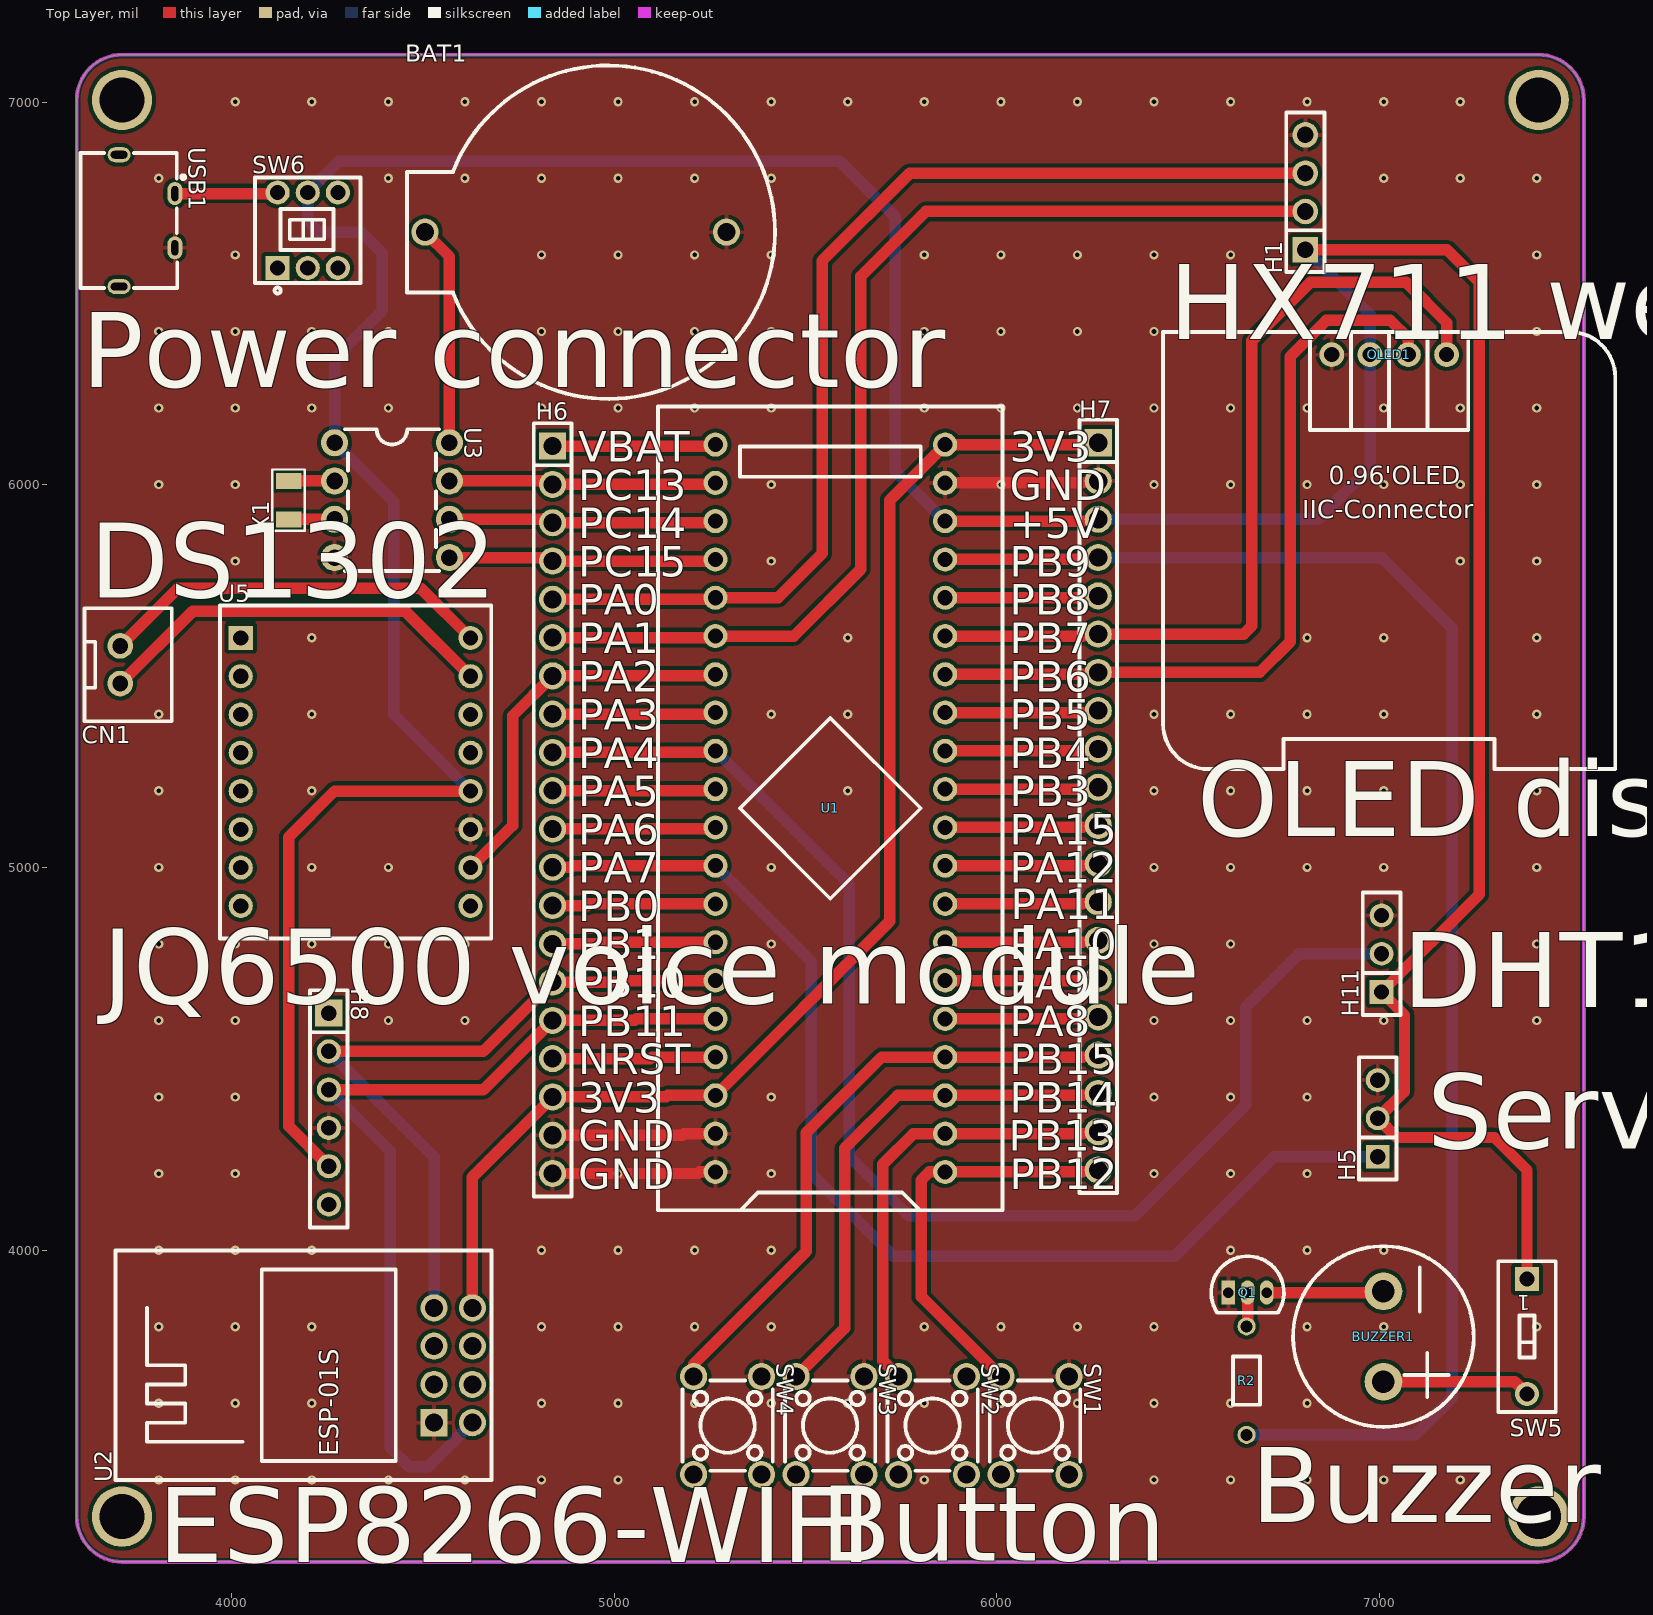
[diagram p0: Top Layer view]
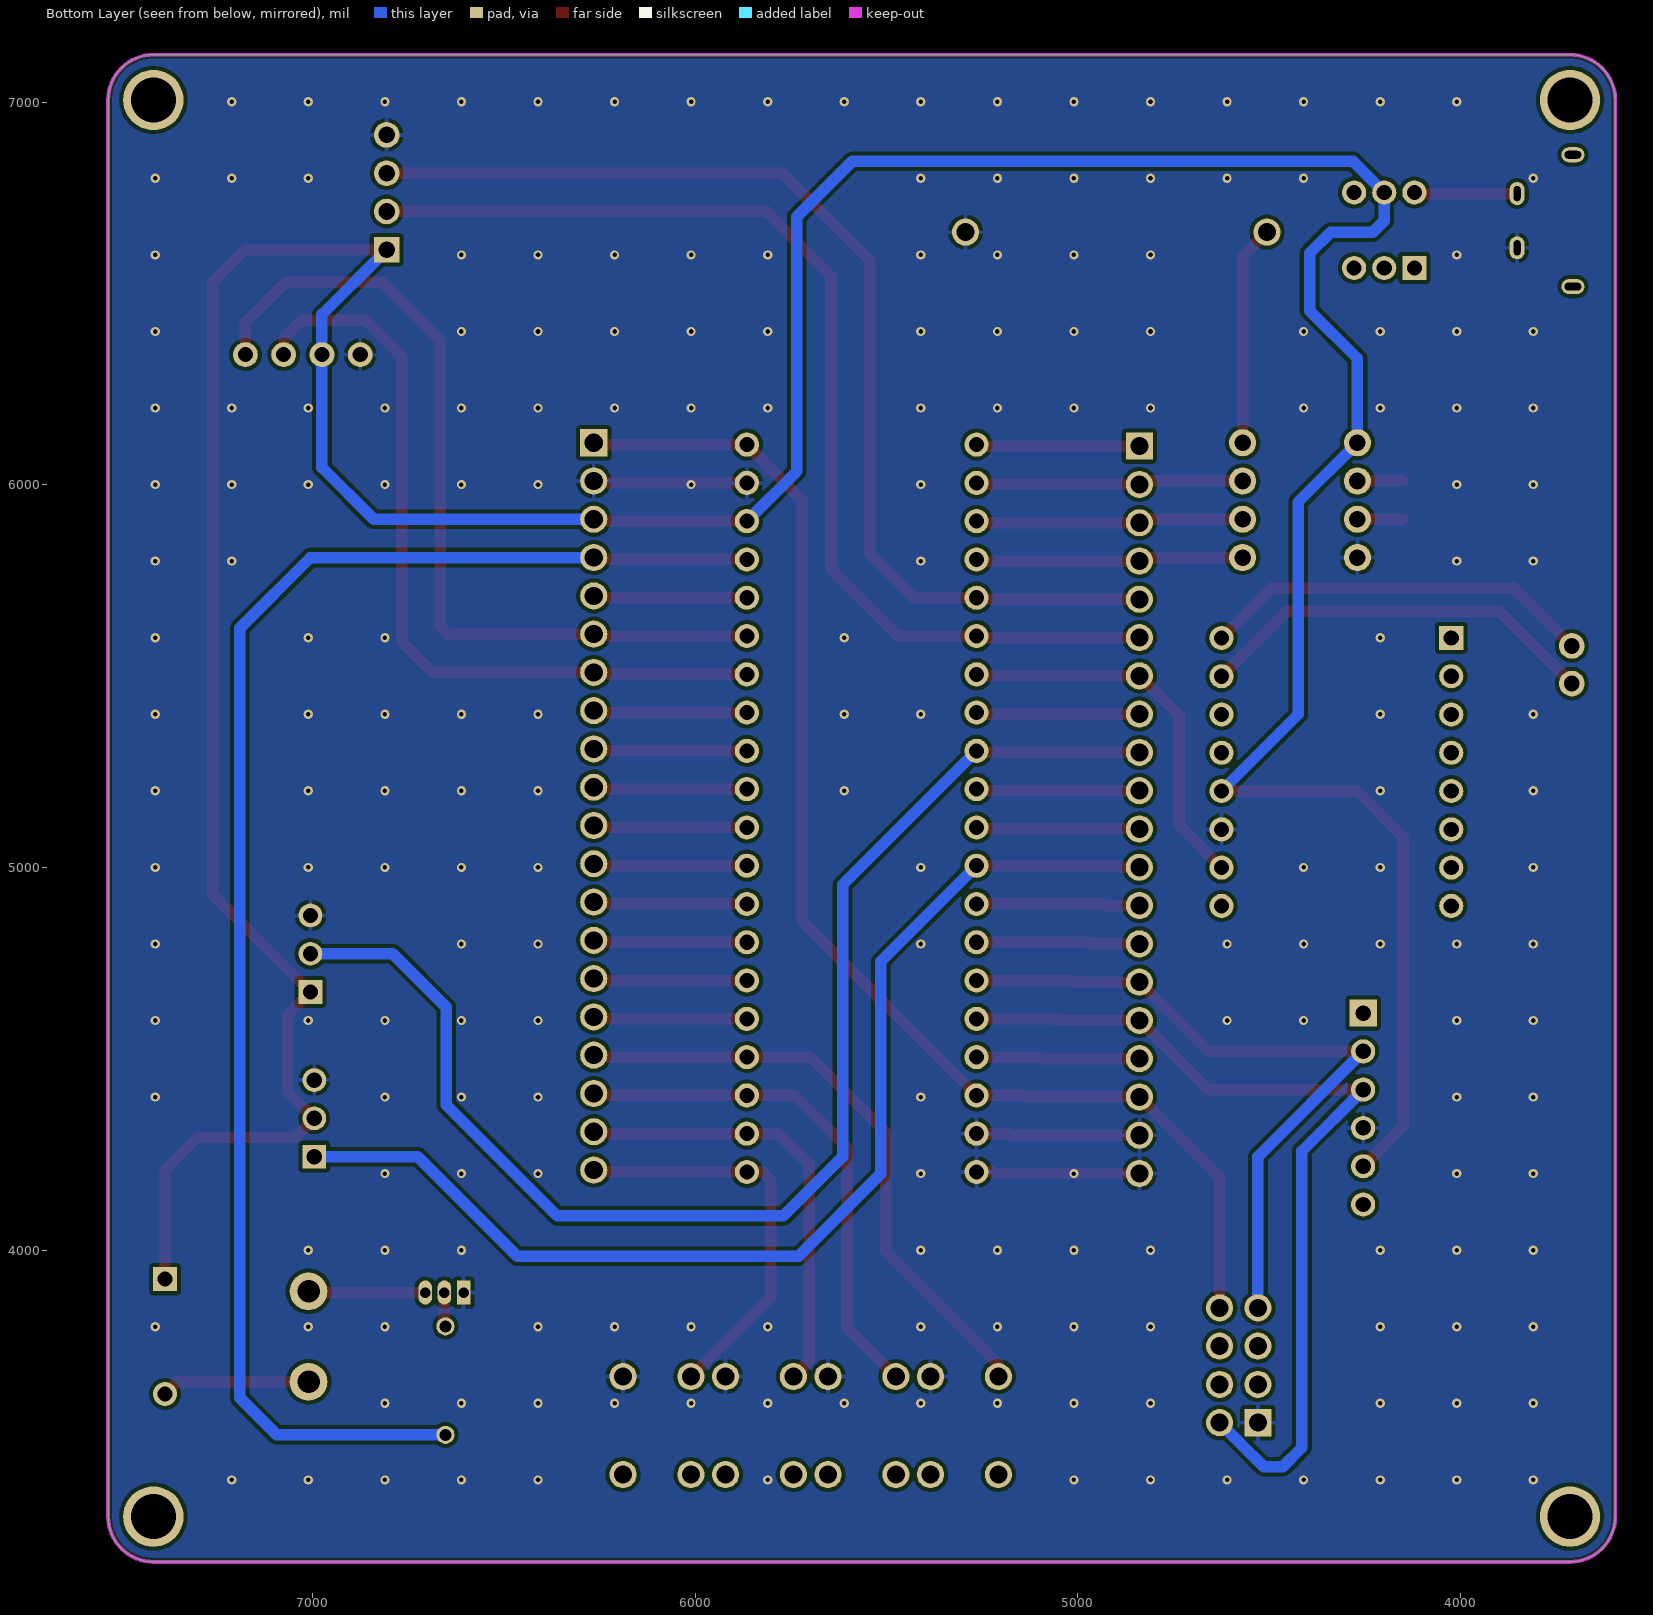
[diagram p1: Bottom Layer view, seen from below]
# Altium PCB MISC51988.pcbdoc
Units mil, origin at the board's own origin, x right, y up, seen from the top; angles counter-clockwise.
Board outline 3937.01 x 3937.01 mil, 2 copper layers (Top Layer, Bottom Layer), stack 62.206 mil thick; 24 components, 46 nets, 177 pads, 198 vias.

## Layer stack, top to bottom
Top Solder Mask Layer: solder mask 0.394, Dk 3.3
Top Layer: signal copper 1.379
Dielectric1: surface 59.449, FR4, Dk 4.5
Bottom Layer: signal copper 1.378
Bottom Solder Mask Layer: solder mask 0.394, Dk 3.3

## Board outline
3714.61,7123.5 ccw(c3714.61,7005.39) 3596.5,7005.39 3596.5,3304.61 ccw(c3714.61,3304.61) 3714.61,3186.5 7415.39,3186.5 ccw(c7415.39,3304.61) 7533.5,3304.61 7533.5,7005.39 ccw(c7415.39,7005.39) 7415.39,7123.5 3714.61,7123.5

## Design rules (kind name [scope] priority, off if disabled: settings)
BoardOutlineClearance copperThickness2oz_1 [All] p2 off: genericclearance=7.99 ignorepadtopadclearanceinfootprint=FALSE except(0: Arc-SplitContinuation Track-SplitContinuation SMDPad-SplitContinuation THPad-SplitContinuation Via-SplitContinuation Fill-SplitContinuation Region-SplitContinuation Poly-SplitContinuation Text-SplitContinuation Hole-SplitContinuation; 5.98: Arc-CutoutEdge Track-CutoutEdge SMDPad-CutoutEdge THPad-CutoutEdge Via-CutoutEdge Text-CutoutEdge; 6.9: Hole-OutlineEdge Hole-CutoutEdge; 10: Poly-OutlineEdge Poly-CutoutEdge; 11.81: Arc-OutlineEdge Track-OutlineEdge SMDPad-OutlineEdge THPad-OutlineEdge Via-OutlineEdge Fill-OutlineEdge Region-OutlineEdge Text-OutlineEdge Fill-CutoutEdge Region-CutoutEdge)
BoardOutlineClearance Plane_innerPlane_1 [All] p4 off: genericclearance=4.02 ignorepadtopadclearanceinfootprint=FALSE except(0: Arc-SplitContinuation Track-SplitContinuation SMDPad-SplitContinuation THPad-SplitContinuation Via-SplitContinuation Fill-SplitContinuation Region-SplitContinuation Poly-SplitContinuation Text-SplitContinuation Hole-SplitContinuation; 5.98: Arc-CutoutEdge Track-CutoutEdge SMDPad-CutoutEdge THPad-CutoutEdge Via-CutoutEdge Text-CutoutEdge; 6.9: Hole-OutlineEdge Hole-CutoutEdge; 10: Poly-OutlineEdge Poly-CutoutEdge; 11.81: Arc-OutlineEdge Track-OutlineEdge SMDPad-OutlineEdge THPad-OutlineEdge Via-OutlineEdge Fill-OutlineEdge Region-OutlineEdge Text-OutlineEdge Fill-CutoutEdge Region-CutoutEdge)
BoardOutlineClearance Copper_copperRegion_1 [All] p6 off: genericclearance=4.02 ignorepadtopadclearanceinfootprint=FALSE except(0: Arc-SplitContinuation Track-SplitContinuation SMDPad-SplitContinuation THPad-SplitContinuation Via-SplitContinuation Fill-SplitContinuation Region-SplitContinuation Poly-SplitContinuation Text-SplitContinuation Hole-SplitContinuation; 5.98: Arc-CutoutEdge Track-CutoutEdge SMDPad-CutoutEdge THPad-CutoutEdge Via-CutoutEdge Text-CutoutEdge; 6.9: Hole-OutlineEdge Hole-CutoutEdge; 10: Poly-OutlineEdge Poly-CutoutEdge; 11.81: Arc-OutlineEdge Track-OutlineEdge SMDPad-OutlineEdge THPad-OutlineEdge Via-OutlineEdge Fill-OutlineEdge Region-OutlineEdge Text-OutlineEdge Fill-CutoutEdge Region-CutoutEdge)
BoardOutlineClearance Copper_copperRegion_copperThickness1oz_1 [All] p8 off: genericclearance=4.02 ignorepadtopadclearanceinfootprint=FALSE except(0: Arc-SplitContinuation Track-SplitContinuation SMDPad-SplitContinuation THPad-SplitContinuation Via-SplitContinuation Fill-SplitContinuation Region-SplitContinuation Poly-SplitContinuation Text-SplitContinuation Hole-SplitContinuation; 5.98: Arc-CutoutEdge Track-CutoutEdge SMDPad-CutoutEdge THPad-CutoutEdge Via-CutoutEdge Text-CutoutEdge; 6.9: Hole-OutlineEdge Hole-CutoutEdge; 10: Poly-OutlineEdge Poly-CutoutEdge; 11.81: Arc-OutlineEdge Track-OutlineEdge SMDPad-OutlineEdge THPad-OutlineEdge Via-OutlineEdge Fill-OutlineEdge Region-OutlineEdge Text-OutlineEdge Fill-CutoutEdge Region-CutoutEdge)
BoardOutlineClearance Copper_copperRegion_Copper_copperRegion_1 [All] p10 off: genericclearance=4.02 ignorepadtopadclearanceinfootprint=FALSE except(0: Arc-SplitContinuation Track-SplitContinuation SMDPad-SplitContinuation THPad-SplitContinuation Via-SplitContinuation Fill-SplitContinuation Region-SplitContinuation Poly-SplitContinuation Text-SplitContinuation Hole-SplitContinuation; 5.98: Arc-CutoutEdge Track-CutoutEdge SMDPad-CutoutEdge THPad-CutoutEdge Via-CutoutEdge Text-CutoutEdge; 6.9: Hole-OutlineEdge Hole-CutoutEdge; 10: Poly-OutlineEdge Poly-CutoutEdge; 11.81: Arc-OutlineEdge Track-OutlineEdge SMDPad-OutlineEdge THPad-OutlineEdge Via-OutlineEdge Fill-OutlineEdge Region-OutlineEdge Text-OutlineEdge Fill-CutoutEdge Region-CutoutEdge)
BoardOutlineClearance copperThickness1oz_1 [All] p12: genericclearance=4.02 ignorepadtopadclearanceinfootprint=FALSE except(0: Arc-SplitContinuation Track-SplitContinuation SMDPad-SplitContinuation THPad-SplitContinuation Via-SplitContinuation Fill-SplitContinuation Region-SplitContinuation Poly-SplitContinuation Text-SplitContinuation Hole-SplitContinuation; 5.98: Arc-CutoutEdge Track-CutoutEdge SMDPad-CutoutEdge THPad-CutoutEdge Via-CutoutEdge Text-CutoutEdge; 6.9: Hole-OutlineEdge Hole-CutoutEdge; 10: Poly-OutlineEdge Poly-CutoutEdge; 11.81: Arc-OutlineEdge Track-OutlineEdge SMDPad-OutlineEdge THPad-OutlineEdge Via-OutlineEdge Fill-OutlineEdge Region-OutlineEdge Text-OutlineEdge Fill-CutoutEdge Region-CutoutEdge)
Clearance copperThickness2oz [All] p1 off: gap=7.99 ignorepadtopadclearanceinfootprint=FALSE except(5.98: SMDPad-Track SMDPad-SMDPad THPad-Track SMDPad-THPad THPad-THPad Track-Via SMDPad-Via THPad-Via Via-Via Fill-SMDPad Region-SMDPad Fill-THPad Region-THPad Fill-Via Region-Via Fill-Fill Fill-Region Region-Region Arc-Track Arc-SMDPad Arc-THPad Arc-Via Fill-Arc Region-Arc Arc-Arc Text-Track SMDPad-Text Text-THPad Text-Via Fill-Text Region-Text Arc-Text Text-Text; 6.9: Hole-Track Hole-SMDPad Hole-THPad Hole-Via Fill-Hole Region-Hole Hole-Arc Hole-Text; 10: Poly-Track Poly-SMDPad Poly-THPad Poly-Via Poly-Fill Poly-Region Poly-Poly Poly-Arc Poly-Text Poly-Hole; 11.81: Fill-Track Region-Track)
Clearance Plane_innerPlane [All] p3 off: gap=4.02 ignorepadtopadclearanceinfootprint=FALSE except(5.98: SMDPad-Track SMDPad-SMDPad THPad-Track SMDPad-THPad THPad-THPad Track-Via SMDPad-Via THPad-Via Via-Via Fill-SMDPad Region-SMDPad Fill-THPad Region-THPad Fill-Via Region-Via Fill-Fill Fill-Region Region-Region Arc-Track Arc-SMDPad Arc-THPad Arc-Via Fill-Arc Region-Arc Arc-Arc Text-Track SMDPad-Text Text-THPad Text-Via Fill-Text Region-Text Arc-Text Text-Text; 6.9: Hole-Track Hole-SMDPad Hole-THPad Hole-Via Fill-Hole Region-Hole Hole-Arc Hole-Text; 10: Poly-Track Poly-SMDPad Poly-THPad Poly-Via Poly-Fill Poly-Region Poly-Poly Poly-Arc Poly-Text Poly-Hole; 11.81: Fill-Track Region-Track)
Clearance Copper_copperRegion [All] p5 off: gap=4.02 ignorepadtopadclearanceinfootprint=FALSE except(5.98: SMDPad-Track SMDPad-SMDPad THPad-Track SMDPad-THPad THPad-THPad Track-Via SMDPad-Via THPad-Via Via-Via Fill-SMDPad Region-SMDPad Fill-THPad Region-THPad Fill-Via Region-Via Fill-Fill Fill-Region Region-Region Arc-Track Arc-SMDPad Arc-THPad Arc-Via Fill-Arc Region-Arc Arc-Arc Text-Track SMDPad-Text Text-THPad Text-Via Fill-Text Region-Text Arc-Text Text-Text; 6.9: Hole-Track Hole-SMDPad Hole-THPad Hole-Via Fill-Hole Region-Hole Hole-Arc Hole-Text; 10: Poly-Track Poly-SMDPad Poly-THPad Poly-Via Poly-Fill Poly-Region Poly-Poly Poly-Arc Poly-Text Poly-Hole; 11.81: Fill-Track Region-Track)
Clearance Copper_copperRegion_copperThickness1oz [All] p7 off: gap=4.02 ignorepadtopadclearanceinfootprint=FALSE except(5.98: SMDPad-Track SMDPad-SMDPad THPad-Track SMDPad-THPad THPad-THPad Track-Via SMDPad-Via THPad-Via Via-Via Fill-SMDPad Region-SMDPad Fill-THPad Region-THPad Fill-Via Region-Via Fill-Fill Fill-Region Region-Region Arc-Track Arc-SMDPad Arc-THPad Arc-Via Fill-Arc Region-Arc Arc-Arc Text-Track SMDPad-Text Text-THPad Text-Via Fill-Text Region-Text Arc-Text Text-Text; 6.9: Hole-Track Hole-SMDPad Hole-THPad Hole-Via Fill-Hole Region-Hole Hole-Arc Hole-Text; 10: Poly-Track Poly-SMDPad Poly-THPad Poly-Via Poly-Fill Poly-Region Poly-Poly Poly-Arc Poly-Text Poly-Hole; 11.81: Fill-Track Region-Track)
Clearance Copper_copperRegion_Copper_copperRegion [All] p9 off: gap=4.02 ignorepadtopadclearanceinfootprint=FALSE except(5.98: SMDPad-Track SMDPad-SMDPad THPad-Track SMDPad-THPad THPad-THPad Track-Via SMDPad-Via THPad-Via Via-Via Fill-SMDPad Region-SMDPad Fill-THPad Region-THPad Fill-Via Region-Via Fill-Fill Fill-Region Region-Region Arc-Track Arc-SMDPad Arc-THPad Arc-Via Fill-Arc Region-Arc Arc-Arc Text-Track SMDPad-Text Text-THPad Text-Via Fill-Text Region-Text Arc-Text Text-Text; 6.9: Hole-Track Hole-SMDPad Hole-THPad Hole-Via Fill-Hole Region-Hole Hole-Arc Hole-Text; 10: Poly-Track Poly-SMDPad Poly-THPad Poly-Via Poly-Fill Poly-Region Poly-Poly Poly-Arc Poly-Text Poly-Hole; 11.81: Fill-Track Region-Track)
Clearance copperThickness1oz [All] p11: gap=4.02 ignorepadtopadclearanceinfootprint=FALSE except(5.98: SMDPad-Track SMDPad-SMDPad THPad-Track SMDPad-THPad THPad-THPad Track-Via SMDPad-Via THPad-Via Via-Via Fill-SMDPad Region-SMDPad Fill-THPad Region-THPad Fill-Via Region-Via Fill-Fill Fill-Region Region-Region Arc-Track Arc-SMDPad Arc-THPad Arc-Via Fill-Arc Region-Arc Arc-Arc Text-Track SMDPad-Text Text-THPad Text-Via Fill-Text Region-Text Arc-Text Text-Text; 6.9: Hole-Track Hole-SMDPad Hole-THPad Hole-Via Fill-Hole Region-Hole Hole-Arc Hole-Text; 10: Poly-Track Poly-SMDPad Poly-THPad Poly-Via Poly-Fill Poly-Region Poly-Poly Poly-Arc Poly-Text Poly-Hole; 11.81: Fill-Track Region-Track)
DiffPairsRouting differentialPair [All] p1: maxlimit=6 minlimit=6 mostfreqgap=6 toplayer_minwidth=5 toplayer_prefwidth=10 toplayer_maxwidth=100 toplayer_mingap=6 toplayer_prefgap=6 toplayer_maxgap=6 bottomlayer_minwidth=5 bottomlayer_prefwidth=10 bottomlayer_maxwidth=100 bottomlayer_mingap=6 bottomlayer_prefgap=6 bottomlayer_maxgap=6 maxuncoupledlength=10
HoleToHoleClearance otherClearance [All] p1: gap=11.81 allowstackedmicrovias=TRUE
Length netLength [All] p1: minlimit=0 maxlimit=0
PasteMaskExpansion pasteMaskExpansion [All] p1: expansion=0
PlaneConnect innerPlane [All] p1: planeconnectstyle=Relief reliefexpansion=20 reliefentries=4 reliefconductorwidth=10 reliefairgap=10
PolygonConnect copperRegion_copperThickness1oz [All] p1 off: connectstyle=Relief reliefconductorwidth=10 reliefentries=4 polygonreliefangle="90 Angle" airgapwidth=10 via.connectstyle=Relief via.reliefconductorwidth=10 via.reliefentries=4 via.polygonreliefangle="90 Angle" via.airgapwidth=10
PolygonConnect copperRegion_Copper_copperRegion [All] p2 off: connectstyle=Relief reliefconductorwidth=10 reliefentries=4 polygonreliefangle="90 Angle" airgapwidth=10 via.connectstyle=Relief via.reliefconductorwidth=10 via.reliefentries=4 via.polygonreliefangle="90 Angle" via.airgapwidth=10
PolygonConnect copperRegion [All] p3: connectstyle=Relief reliefconductorwidth=10 reliefentries=4 polygonreliefangle="90 Angle" airgapwidth=10 via.connectstyle=Relief via.reliefconductorwidth=10 via.reliefentries=4 via.polygonreliefangle="90 Angle" via.airgapwidth=10
RoutingVias viaSize [All] p1: holewidth=12.01 width=24.02 viastyle="Through Hole" minholewidth=11.81 minwidth=19.68 maxholewidth=248.03 maxwidth=393.7
SolderMaskExpansion solderMaskExpansion [IsVia] p1: expansion=-1000 istentingtop=TRUE
SolderMaskExpansion solderMaskExpansion [All] p2: expansion=2 istentingtop=FALSE
Width copperThickness2oz_2 [All] p1 off: maxlimit=100 minlimit=8 preferedwidth=10
Width copperThickness1oz_2 [All] p2: maxlimit=100 minlimit=5 preferedwidth=10

## Components (designator, comment, footprint, x,y, rotation, side; value= is the part's Value field where it differs from the comment)
BAT1 "KH-BS2032-2-1" BAT-TH_KH-BS2032-2-1 4900,6660 r0 top
BUZZER1 "buzzer" BUZ-TH_BD12.0-P6.00-D0.9-RD 7010,3775 r270 top
CN1 "XH2.54*2P_Through-hole" CONN-TH_2P-P2.50-XH2.54-2P 3710,5530 r90 top
H1 "" HDR-TH_4P-P2.54-V-F 6806.03,6764.04 r90 top
H5 "" HDR-TH_3P-P2.54-V-F 6995,4345 r90 top
H6 "" HDR-TH_20P-P2.54-V-F 4839.74,5150.95 r270 top
H7 "" HDR-TH_20P-P2.54-V-F 6265,5160 r270 top
H8 "" HDR-TH_6P-P2.54-V-F 4255,4370 r270 top
H11 "" HDR-TH_3P-P2.54-V-F 7005,4775 r90 top
OLED1 "" 0.96OLED_4P 7025,6340 r0 top
Q1 "" S8050_TO_92 6655,3890 r0 top
R2 "1kΩ" Res_1/8W 6655,3660 r90 top
SW1 "" SW-TH_4P-L6.0-W6.0-P4.50-LS6.5 6099.85,3542.47 r270 top
SW2 "" SW-TH_4P-L6.0-W6.0-P4.50-LS6.5 5832.14,3542.47 r270 top
SW3 "" SW-TH_4P-L6.0-W6.0-P4.50-LS6.5 5564.43,3542.47 r270 top
SW4 "" SW-TH_4P-L6.0-W6.0-P4.50-LS6.5 5296.72,3542.47 r270 top
SW5 "NDS-01V" SW-TH_2P-L3.9-W9.9-P2.54-LS7.6 7385,3775 r270 top
SW6 "TK-6700-1" SW-TH_TK-6700-1 4200,6665 r0 top
U1 "STM32F103C8T6-Card" CONN-TH_L53.3-W22.9_STM32F103C8T6-CARD 5565,5155 r90 top
U2 "ESP-01S" WIFIM-TH_ESP-01S 4580,3700 r90 top
U3 "DS1302N(XBLW)" PDIP-8_L9.3-W6.4-P2.54-LS7.6-BL 4420,5960 r270 top
U5 "JQ6500" MOD-TH_JQ6500 4325,5250 r0 top
USB1 "KH-TYPE-C-2P" USB-SMD_KH-TYPE-C-2P 3780,6690 r270 top
X1 "32.768KHZ" CRYSTAL-SMD_L3.2-W1.5-1 4150,5960 r90 top

## Footprints (in the part's own frame and the unit in brackets; to place one, negate y for a bottom-side part, rotate by r counter-clockwise, add the part's x,y. Pads: shape width x height; smd on the part's side, far side on the other; paste and mask are expansions set on the pad)
0.96OLED_4P [mm]
  round 1.65 hole 1 copper offset 0,0: 1(-3.81,-0.001) 2(-1.27,0.002) 3(1.27,0.002) 4(3.81,0.002)
  silkscreen extent -15,-27.5 15,1.5
BAT-TH_KH-BS2032-2-1 [mm]
  round 1.8 hole 1.2 paste+0 mask+0.05: 1(-10,0) 2(10,0)
  silkscreen extent -11.2,-11.06 13.22,11.06
BUZ-TH_BD12.0-P6.00-D0.9-RD [mm]
  round 2.5 hole 1.5 paste+0 mask+0.05: 1(-3,0) 2(3,0)
  silkscreen extent -5.99,-5.99 5.99,5.99
CONN-TH_2P-P2.50-XH2.54-2P [mm]
  round 1.7 hole 1.05 paste+0 mask+0.05: 1(1.25,0) 2(-1.25,0)
  silkscreen extent -3.75,-3.42 3.75,2.37
CONN-TH_L53.3-W22.9_STM32F103C8T6-CARD [mm]
  round 1.6 hole 1: 1(-24.13,-7.62) 2(-21.59,-7.62) 3(-19.05,-7.62) 4(-16.51,-7.62) 5(-13.97,-7.62) 6(-11.43,-7.62) 7(-8.89,-7.62) 8(-6.35,-7.62) 9(-3.81,-7.62) 10(-1.27,-7.62) 11(1.27,-7.62) 12(3.81,-7.62) 13(6.35,-7.62) 14(8.89,-7.62) 15(11.43,-7.62) 16(13.97,-7.62) 17(16.51,-7.62) 18(19.05,-7.62) 19(21.59,-7.62) 20(24.13,-7.62) 21(24.13,7.62) 22(21.59,7.62) 23(19.05,7.62) 24(16.51,7.62) 25(13.97,7.62) 26(11.43,7.62) 27(8.89,7.62) 28(6.35,7.62) 29(3.81,7.62) 30(1.27,7.62) 31(-1.27,7.62) 32(-3.81,7.62) 33(-6.35,7.62) 34(-8.89,7.62) 35(-11.43,7.62) 36(-13.97,7.62) 37(-16.51,7.62) 38(-19.05,7.62) 39(-21.59,7.62) 40(-24.13,7.62)
  silkscreen extent -26.67,-11.43 26.67,11.43
CRYSTAL-SMD_L3.2-W1.5-1 [mm]
  rect 1.05x1.7 smd: 1(-1.275,0) 2(1.275,0)
  silkscreen extent -2.03,-1.08 2.03,1.08
HDR-TH_3P-P2.54-V-F [mil]
  rect 62x62 hole 40.16: 1(-100,0)
  round 62 hole 40.16: 2(0,0) 3(100,0)
  silkscreen extent -160,-49 160,49
HDR-TH_4P-P2.54-V-F [mm]
  rect 1.7x1.7 hole 1.1: 1(-3.81,0)
  round 1.7 hole 1.1: 2(-1.27,0) 3(1.27,0) 4(3.81,0)
  silkscreen extent -5.29,-1.27 5.29,1.27
HDR-TH_6P-P2.54-V-F [mm]
  rect 1.8x1.8 hole 1.02: 1(-6.35,0)
  round 1.6 hole 1.02: 2(-3.81,0) 3(-1.27,0) 4(1.27,0) 5(3.81,0) 6(6.35,0)
  silkscreen extent -7.87,-1.25 7.87,1.25
HDR-TH_20P-P2.54-V-F [mm]
  rect 1.8x1.8 hole 1.2: 1(-24.13,0)
  round 1.8 hole 1.2: 2(-21.59,0) 3(-19.05,0) 4(-16.51,0) 5(-13.97,0) 6(-11.43,0) 7(-8.89,0) 8(-6.35,0) 9(-3.81,0) 10(-1.27,0) 11(1.27,0) 12(3.81,0) 13(6.35,0) 14(8.89,0) 15(11.43,0) 16(13.97,0) 17(16.51,0) 18(19.05,0) 19(21.59,0) 20(24.13,0)
  silkscreen extent -25.65,-1.25 25.65,1.25
MOD-TH_JQ6500 [mm]
  rect 1.6x1.6 hole 1: 1(-7.62,8.89)
  round 1.6 hole 1: 2(-7.62,6.35) 3(-7.62,3.81) 4(-7.62,1.27) 5(-7.62,-1.27) 6(-7.62,-3.81) 7(-7.62,-6.35) 8(-7.62,-8.89) 9(7.62,-8.89) 10(7.62,-6.35) 11(7.62,-3.81) 12(7.62,-1.27) 13(7.62,1.27) 14(7.62,3.81) 15(7.62,6.35) 16(7.62,8.89)
  silkscreen extent -9,-11.05 9,11.05
PDIP-8_L9.3-W6.4-P2.54-LS7.6-BL [mm]
  round 1.8 hole 1.1: 1(-3.81,-3.81) 2(-1.27,-3.81) 3(1.27,-3.81) 4(3.81,-3.81) 5(3.81,3.81) 6(1.27,3.81) 7(-1.27,3.81) 8(-3.81,3.81)
  silkscreen extent -4.7,-3.11 4.7,3.11
Res_1/8W [mil]
  round 47.2 hole 31.5 paste+0 mask+2: 1(-141.7,2.48) 2(141.7,2.48)
  silkscreen extent -63,-33 63,38
S8050_TO_92 [mil]
  rect 35.4x63 hole 27.6 paste+0 mask+2: 1(-50,0)
  oval 35.4x63 hole 27.6 paste+0 mask+2: 2(0,0) 3(50,0)
  silkscreen extent -95,-53 95,95
SW-TH_2P-L3.9-W9.9-P2.54-LS7.6 [mm]
  rect 1.6x1.6 hole 1 paste+0 mask+0.05: 1(-3.81,0)
  round 1.6 hole 1 paste+0 mask+0.05: 2(3.81,0)
  silkscreen extent -5,-1.91 5,1.91
SW-TH_4P-L6.0-W6.0-P4.50-LS6.5 [mm]
  round 1.8 hole 1.2: 1(-3.25,2.25) 2(3.25,2.25) 3(-3.25,-2.25) 4(3.25,-2.25)
  silkscreen extent -3,-3 3,3
SW-TH_TK-6700-1 [mm]
  rect 1.6x1.6 hole 1: 1(-2,-2.5)
  round 1.6 hole 1: 2(0,-2.5) 3(2,-2.5)
  round 1.6 hole 1 copper offset 0,0: 4(-2,2.5) 5(0,2.5) 6(2,2.5)
  silkscreen extent -3.5,-4.2 3.5,3.5
USB-SMD_KH-TYPE-C-2P [mm]
  oval 1.524x1 hole 0.45 slot 1 at 0 deg paste+0 mask+0.05: 1(-1.8,1.85) 2(1.8,1.85)
  oval 1x1.524 hole 0.5 slot 1.1 at 90 deg paste+0 mask+0.05: 3(4.375,-1.85) 4(-4.375,-1.85)
  silkscreen extent -4.5,-4.41 4.46,2.53
WIFIM-TH_ESP-01S [mm]
  rect 1.8x1.8 hole 1.2: 1(-3.81,1.27)
  round 1.8 hole 1.2: 2(-1.27,1.27) 3(1.27,1.27) 4(3.81,1.27) 5(3.81,-1.27) 6(1.27,-1.27) 7(-1.27,-1.27) 8(-3.81,-1.27)
  silkscreen extent -7.62,-2.54 7.62,22.4

## Free pads (board coordinates)
  round 157.48 hole 118.11: 1(3714.61,7005.39) 1(3714.61,3304.61) 1(7415.39,7005.39) 1(7415.39,3304.61)

## Via types
v1: diameter 24.02, hole 12, Top Layer to Bottom Layer, 198 vias

## Nets (pads, with @x,y where several pads share a name; then routed paths per layer and width w, separated by ;. In a path a pad name is that pad's centre, name@x,y a point inside that pad or via, vN(x,y) a via of type N, cw(c..) or ccw(c..) an arc to the next point about the centre after c; other vN are vias at no path point)
3V3: H6.18 H7.1 U1.20 U1.38 U2.5 | length 3373.3
  Top Layer w30: U2.5 4630,4191.21 H6.18 5136.61,4400.95 5140.66,4405 U1.38 5720,4860 5720,5960 U1.20 6225,6105
$1N1498: H7.16 U1.5 | length 360
  Top Layer w30: U1.5 6225,4605
$1N1504: H7.13 U1.8 | length 360
  Top Layer w30: U1.8 6225,4905
$1N1506: H7.12 U1.9 | length 360
  Top Layer w30: U1.9 6225,5005
$1N1508: H7.11 U1.10 | length 360
  Top Layer w30: U1.10 6225,5105
$1N1510: H7.10 U1.11 | length 360
  Top Layer w30: U1.11 6225,5205
$1N1512: H7.9 U1.12 | length 360
  Top Layer w30: U1.12 6225,5305
$1N1514: H7.8 U1.13 | length 360
  Top Layer w30: U1.13 6225,5405
$1N1520: H7.5 U1.16 | length 360
  Top Layer w30: U1.16 6225,5705
$1N1548: H6.10 U1.30 | length 426.9
  Top Layer w30: H6.10 5260.95,5200.95 U1.30
$1N1550: H6.11 U1.31 | length 426.9
  Top Layer w30: H6.11 5260.95,5100.95 U1.31
$1N1554: H6.13 U1.33 | length 426.9
  Top Layer w30: H6.13 4929.5,4900.95 4933.55,4905 U1.33
$1N1556: H6.14 U1.34 | length 426.9
  Top Layer w30: H6.14 4970.92,4800.95 4974.97,4805 U1.34
$1N1562: H6.17 U1.37 | length 426.9
  Top Layer w30: H6.17 5095.19,4500.95 5099.24,4505 U1.37
$1N17183: BAT1.1 U3.8 | length 576.4
  Top Layer w30: BAT1.1 4570,6596.3 U3.8
$1N17188: U3.2 X1.2 | length 120.1
  Top Layer w30: X1.2 4150.2,6010 U3.2
$1N17190: U3.3 X1.1 | length 120.1
  Top Layer w30: X1.1 4269.8,5909.8 U3.3
$1N17200: CN1.1 U5.16 | length 1031.3
  Top Layer w30: CN1.1 3860.78,5730 4495,5730 U5.16
$1N17201: CN1.2 U5.15 | length 1063.8
  Top Layer w30: CN1.2 3899.22,5670 4455,5670 U5.15
$1N17205: Q1.2 R2.2 | length 89.3
  Top Layer w30: R2.2 6655,3804.18 Q1.2
$1N17207: BUZZER1.2 SW5.2 | length 388.2
  Top Layer w30: BUZZER1.2 7353.11,3656.89 SW5.2
$1N17208: BUZZER1.1 Q1.3 | length 306.3
  Top Layer w30: Q1.3 7006.89,3890 BUZZER1.1
+5V: H1.1 H5.2 H7.3 H8.5 H11.1 OLED1.2 SW5.1 SW6.5 U1.18 U3.1 U5.12 | length 11142.5
  Top Layer w30: H8.5 4150,4325 4150,5080 4270,5200 U5.12 ; U1.18 6225,5905 ; H1.1 7175.96,6614.04 7260,6530 7260,4930 H11.1 7065,4615 7065,4415 H5.2 7045,4295 7300,4295 7385,4210 SW5.1
  Bottom Layer w30: U5.12 4425,5400 4425,5955 U3.1 4270,6330 4395,6455 4395,6605 4340,6660 4230,6660 4200,6690 SW6.5 4281.58,6845 5590,6845 5735,6700 5735,6035 U1.18 ; H7.3 6840,5910 6975,6045 6975,6340.05 6975,6445.07 H1.1
DAT: H1.3 H6.5 U1.25 | length 2875.5
  Top Layer w30: H6.5 5260.95,5700.95 U1.25 5428.58,5705 5544.29,5820.71 5544.29,6585.71 5772.62,6814.04 H1.3
GND: BAT1.2 H1.4 H5.3 H6.19 H6.20 H7.2 H8.4 H11.3 OLED1.1 Q1.1 SW1.1 SW2.1 SW3.1 SW4.1 U1.19 U1.39 U1.40 U2.1 U3.4 U5.11 USB1.2 | length 1213.9
  Top Layer w30: H6.20 5219.45,4200.95 5223.5,4205 U1.40 ; H6.19 5178.03,4300.95 5182.08,4305 U1.39 ; U1.19 6225,6005
  other v1: 3810.6,3400.6 4010.6,3400.6 4210.6,3400.6 4410.6,3400.6 4610.6,3400.6 4810.6,3400.6 5010.6,3400.6 5810.6,3400.6 6410.6,3400.6 6610.6,3400.6 6810.6,3400.6 7010.6,3400.6 7210.6,3400.6 3810.6,3600.6 4010.6,3600.6 4210.6,3600.6 4810.6,3600.6 5010.6,3600.6 5210.6,3600.6 5410.6,3600.6 5610.6,3600.6 5810.6,3600.6 6010.6,3600.6 6210.6,3600.6 6410.6,3600.6 6610.6,3600.6 6810.6,3600.6 3810.6,3800.6 4010.6,3800.6 4210.6,3800.6 4810.6,3800.6 5010.6,3800.6 5210.6,3800.6 5410.6,3800.6 5810.6,3800.6 6010.6,3800.6 6210.6,3800.6 6410.6,3800.6 6810.6,3800.6 7010.6,3800.6 7410.6,3800.6 3810.6,4000.6 4010.6,4000.6 4210.6,4000.6 4810.6,4000.6 5010.6,4000.6 5210.6,4000.6 5410.6,4000.6 6610.6,4000.6 6810.6,4000.6 7010.6,4000.6 3810.6,4200.6 4010.6,4200.6 5010.6,4200.6 5410.6,4200.6 6410.6,4200.6 6610.6,4200.6 6810.6,4200.6 3810.6,4400.6 4010.6,4400.6 5410.6,4400.6 6410.6,4400.6 6610.6,4400.6 6810.6,4400.6 7410.6,4400.6 3810.6,4600.6 4010.6,4600.6 4410.6,4600.6 4610.6,4600.6 6410.6,4600.6 6610.6,4600.6 6810.6,4600.6 7010.6,4600.6 7410.6,4600.6 3810.6,4800.6 4010.6,4800.6 4210.6,4800.6 4410.6,4800.6 4610.6,4800.6 5410.6,4800.6 6410.6,4800.6 6610.6,4800.6 7410.6,4800.6 3810.6,5000.6 4210.6,5000.6 4410.6,5000.6 5410.6,5000.6 6410.6,5000.6 6610.6,5000.6 6810.6,5000.6 7010.6,5000.6 7410.6,5000.6 3810.6,5200.6 4210.6,5200.6 5610.6,5200.6 6410.6,5200.6 6610.6,5200.6 6810.6,5200.6 7010.6,5200.6 7410.6,5200.6 3810.6,5400.6 4210.6,5400.6 5410.6,5400.6 5610.6,5400.6 6410.6,5400.6 6610.6,5400.6 6810.6,5400.6 7010.6,5400.6 7410.6,5400.6 4210.6,5600.6 5610.6,5600.6 6810.6,5600.6 7010.6,5600.6 7410.6,5600.6 3810.6,5800.6 4010.6,5800.6 5410.6,5800.6 7210.6,5800.6 7410.6,5800.6 3810.6,6000.6 4010.6,6000.6 5410.6,6000.6 6010.6,6000.6 6410.6,6000.6 6610.6,6000.6 6810.6,6000.6 7010.6,6000.6 7210.6,6000.6 7410.6,6000.6 3810.6,6200.6 4010.6,6200.6 4210.6,6200.6 4410.6,6200.6 4810.6,6200.6 5010.6,6200.6 5210.6,6200.6 5410.6,6200.6 5810.6,6200.6 6010.6,6200.6 6210.6,6200.6 6410.6,6200.6 6610.6,6200.6 6810.6,6200.6 7010.6,6200.6 7210.6,6200.6 7410.6,6200.6 3810.6,6400.6 4010.6,6400.6 4210.6,6400.6 4410.6,6400.6 4810.6,6400.6 5010.6,6400.6 5210.6,6400.6 5410.6,6400.6 5810.6,6400.6 6010.6,6400.6 6210.6,6400.6 6410.6,6400.6 6610.6,6400.6 7410.6,6400.6 4010.6,6600.6 4810.6,6600.6 5010.6,6600.6 5210.6,6600.6 5410.6,6600.6 5810.6,6600.6 6010.6,6600.6 6210.6,6600.6 6410.6,6600.6 6610.6,6600.6 7410.6,6600.6 3810.6,6800.6 4410.6,6800.6 4610.6,6800.6 4810.6,6800.6 5010.6,6800.6 5210.6,6800.6 5410.6,6800.6 7010.6,6800.6 7210.6,6800.6 7410.6,6800.6 4010.6,7000.6 4210.6,7000.6 4410.6,7000.6 4610.6,7000.6 4810.6,7000.6 5010.6,7000.6 5210.6,7000.6 5410.6,7000.6 5610.6,7000.6 5810.6,7000.6 6010.6,7000.6 6210.6,7000.6 6410.6,7000.6 6610.6,7000.6 6810.6,7000.6 7010.6,7000.6 7210.6,7000.6
PA4: H6.9 H11.2 U1.29 | length 3519.2
  Top Layer w30: H6.9 5260.95,5300.95 U1.29
  Bottom Layer w30: U1.29 5615,4955 5615,4245 5770,4090 6360,4090 6650,4380 6650,4635 6790,4775 H11.2
PA7: H5.1 H6.12 U1.32 | length 3012.2
  Top Layer w30: H6.12 4888.08,5000.95 4892.13,5005 U1.32
  Bottom Layer w30: U1.32 5515,4755 5515,4200 5730,3985 6465,3985 6725,4245 H5.1
PB6: H7.7 OLED1.3 U1.14 | length 2049.3
  Top Layer w30: U1.14 6225,5505 ; H7.7 6686.42,5510 6766.21,5589.79 6766.21,6335 6860.61,6429.39 7028.14,6429.39 7075,6382.53 OLED1.3@7075,6340.05
PB7: H7.6 OLED1.4 U1.15 | length 2214.9
  Top Layer w30: U1.15 6225,5605 ; H7.6 6645,5610 6666.21,5631.21 6666.21,6376.42 6819.19,6529.39 7069.56,6529.39 7175,6423.95 OLED1.4@7175,6340.05
PB9: H7.4 R2.1 U1.17 | length 3949.2
  Top Layer w30: U1.17 6225,5805
  Bottom Layer w30: H7.4 7005,5810 7190,5625 7190,3615 7093.3,3518.3 R2.1
PB12: H7.20 SW1.3 U1.1 | length 1031.4
  Top Layer w30: SW1.3 5802.29,3879.4 5802.29,4183.79 5823.5,4205 U1.1 6225,4205
PB13: H7.19 SW2.3 U1.2 | length 1127.6
  Top Layer w30: SW2.3 5702.29,3711.69 5702.29,4225.21 5782.08,4305 U1.2 6225,4305
PB14: H7.18 SW3.3 U1.3 | length 1328.6
  Top Layer w30: SW3.3 5602.29,3796.86 5602.29,4266.63 5740.66,4405 U1.3 6225,4405
PB15: H7.17 SW4.3 U1.4 | length 1563.8
  Top Layer w30: SW4.3 5208.14,3703.23 5502.29,3997.38 5502.29,4308.05 5699.24,4505 U1.4 6225,4505
PC13: H6.2 U1.22 U3.7 | length 700.4
  Top Layer w30: U3.7 4830.69,6010 H6.2 5260.95,6000.95 U1.22
PC14: H6.3 U1.23 U3.6 | length 700.4
  Top Layer w30: U3.6 4830.69,5910 H6.3 5260.95,5900.95 U1.23
PC15: H6.4 U1.24 U3.5 | length 700.4
  Top Layer w30: U3.5 4830.69,5810 H6.4 5260.95,5800.95 U1.24
SCK: H1.2 H6.6 U1.26 | length 2875.5
  Top Layer w30: H6.6 5260.95,5600.95 U1.26 5470,5605 5644.29,5779.29 5644.29,6544.29 5814.04,6714.04 H1.2
U1_RX: H7.14 U1.7 | length 360
  Top Layer w30: U1.7 6225,4805
U1_TX: H7.15 U1.6 | length 360
  Top Layer w30: U1.6 6225,4705
U2_RX: H6.8 U1.28 | length 426.9
  Top Layer w30: H6.8 5260.95,5400.95 U1.28
U2_TX: H6.7 U1.27 U5.10 | length 1016.8
  Top Layer w30: U5.10 4735,5110 4735,5396.21 H6.7 5260.95,5500.95 U1.27
U3_RX: H6.16 H8.3 U1.36 U2.8 | length 2371.3
  Top Layer w30: H8.3 4658.79,4420 H6.16 5053.77,4600.95 5057.82,4605 U1.36
  Bottom Layer w30: H8.3 4415,4260 4415,3485 4465,3435 4515,3435 4577.18,3497.18 ccw(c4565.43,3514.57) 4582.82,3502.82 U2.8
U3_TX: H6.15 H8.2 U1.35 U2.4 | length 1870.5
  Top Layer w30: H8.2 4658.79,4520 H6.15 5012.34,4700.95 5016.4,4705 U1.35
  Bottom Layer w30: H8.2 4530,4245 U2.4
VBAT: H6.1 U1.21 | length 426.9
  Top Layer w30: H6.1 5260.95,6100.95 U1.21
VUSB: SW6.4 USB1.1 | length 269.5
  Top Layer w30: USB1.1 4118.7,6760.87 SW6.4
pads on no net: H8.1 H8.6 SW1.2 SW1.4 SW2.2 SW2.4 SW3.2 SW3.4 SW4.2 SW4.4 SW6.1 SW6.2 SW6.3 SW6.6 U2.2 U2.3 U2.6 U2.7 U5.1 U5.2 U5.3 U5.4 U5.5 U5.6 U5.7 U5.8 U5.9 U5.13 U5.14 USB1.3 USB1.4

## Polygon pours and split planes (outlines as drawn)
GND on Bottom Layer (solid, remove dead copper, pour order 2): 3525,7245 3525,3080 7700,3080 7700,7245
GND on Top Layer (solid, remove dead copper, pour order 2): 3000,7415 3000,3000 7930,3000 7930,7415

## Keep-outs
Board Outline Layer:
  the board outline again, w10

## Silkscreen, mask and mechanical layers (free items; w line width, h text height)
Top Silkscreen Layer:
  text "HX711 weighing" at 6450,6380 h196.85
  text "Power connector" at 3610,6255 h196.85
  text "VBAT" at 4905.95,6060 h80
  text "3V3" at 6034.16,6060 h80
  text "PC13" at 4905.95,5960 h80
  text "GND" at 6034.16,5960 h80
  text "PC14" at 4905.95,5860 h80
  text "+5V" at 6034.16,5860 h80
  text "PC15" at 4905.95,5760 h80
  text "PB9" at 6034.16,5760 h80
  text "DS1302" at 3630,5705 h196.85
  text "PA0" at 4905.95,5660 h80
  text "PB8" at 6034.16,5660 h80
  text "PA1" at 4905.95,5560 h80
  text "PB7" at 6034.16,5560 h80
  text "PA2" at 4905.95,5460 h80
  text "PB6" at 6034.16,5460 h80
  text "PA3" at 4905.95,5360 h80
  text "PB5" at 6034.16,5360 h80
  text "PA4" at 4905.95,5260 h80
  text "PB4" at 6034.16,5260 h80
  text "PA5" at 4905.95,5160 h80
  text "PB3" at 6034.16,5160 h80
  text "OLED display" at 6523.66,5081.57 h196.85
  text "PA6" at 4905.95,5060 h80
  text "PA15" at 6034.16,5060 h80
  text "PA7" at 4905.95,4960 h80
  text "PA12" at 6034.16,4960 h80
  text "PA11" at 6035.95,4865 h80
  text "PB0" at 4905.95,4860 h80
  text "PB1" at 4905.95,4760 h80
  text "PA10" at 6034.16,4760 h80
  text "PB10" at 4905.95,4660 h80
  text "PA9" at 6034.16,4660 h80
  text "JQ6500 voice module" at 3665,4645 h196.85
  text "DHT11" at 7060,4635 h196.85
  text "PB11" at 4905.95,4560 h80
  text "PA8" at 6034.16,4560 h80
  text "NRST" at 4905.95,4460 h80
  text "PB15" at 6034.16,4460 h80
  text "3V3" at 4905.95,4360 h80
  text "PB14" at 6034.16,4360 h80
  text "Servo" at 7125,4265 h196.85
  text "GND" at 4905.95,4260 h80
  text "PB13" at 6030.95,4260 h80
  text "GND" at 4905.95,4160 h80
  text "PB12" at 6034.16,4160 h80
  text "Buzzer" at 6665,3290 h196.85
  text "Button" at 5540,3190 h196.85
  text "ESP8266-WIFI" at 3810,3185 h196.85